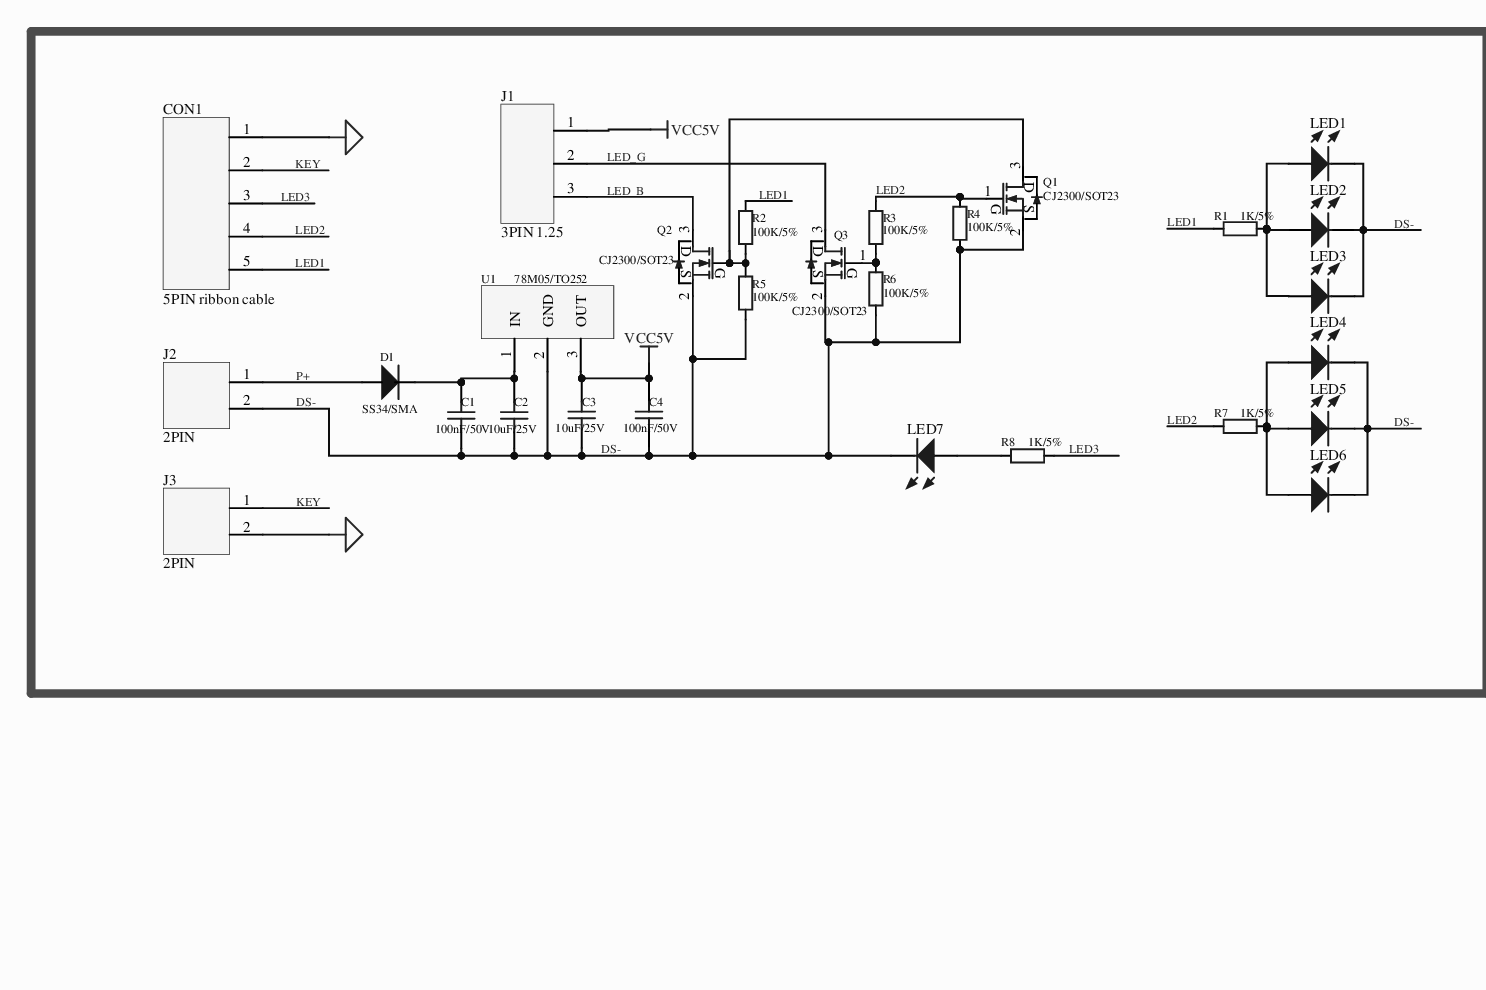
[diagram p0: MISC88840.SchDoc, top left]
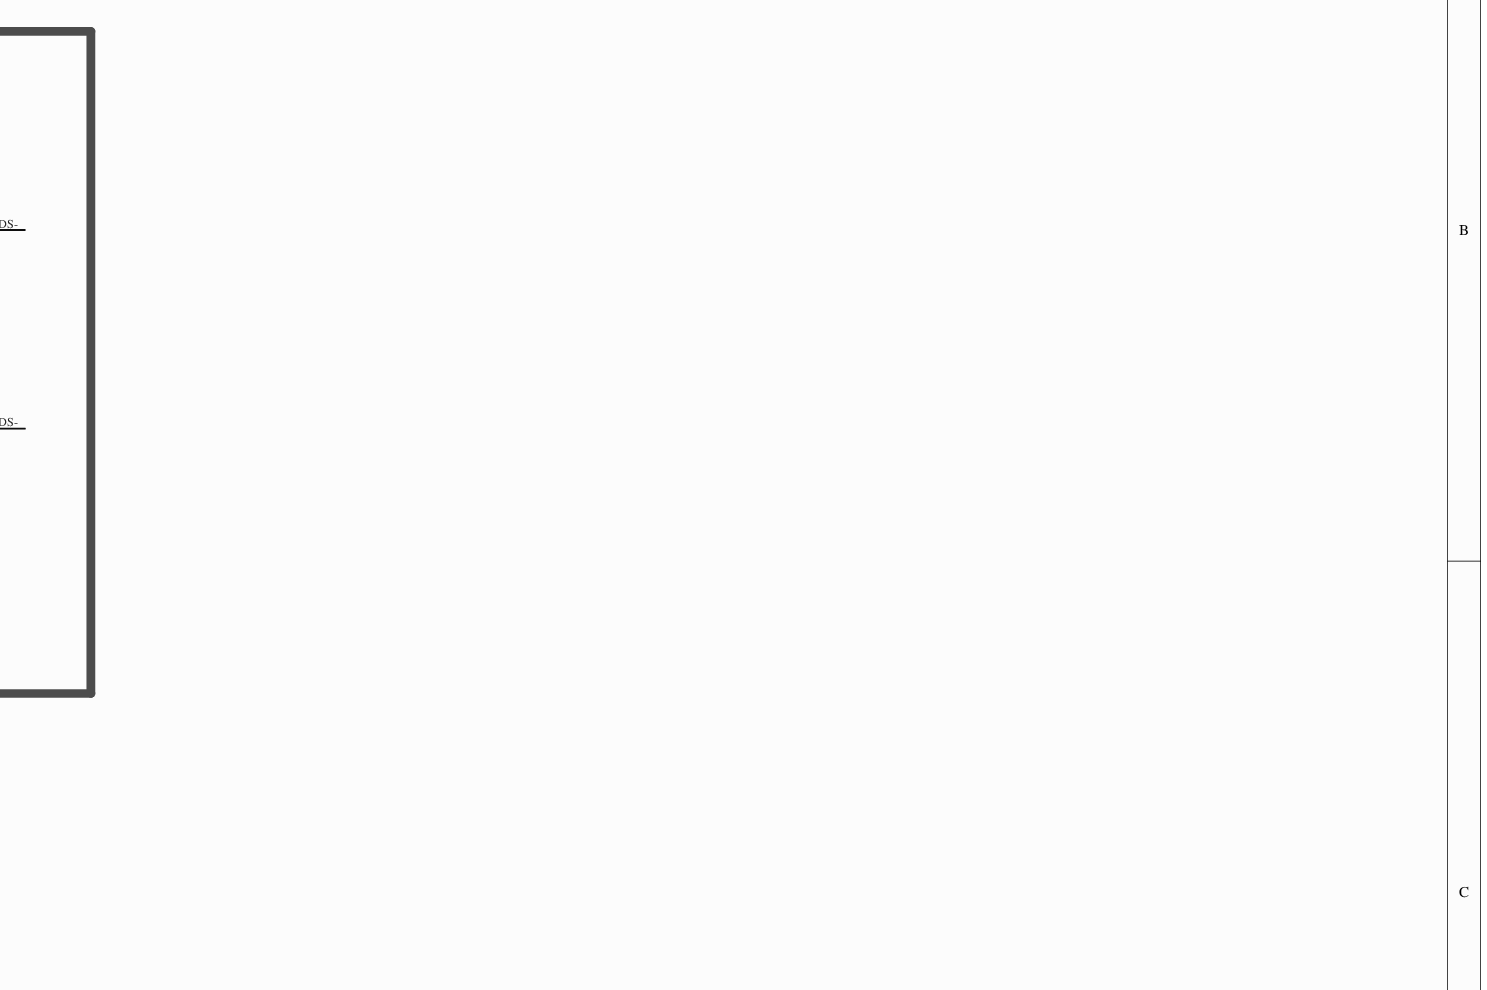
[diagram p1: MISC88840.SchDoc, top right]
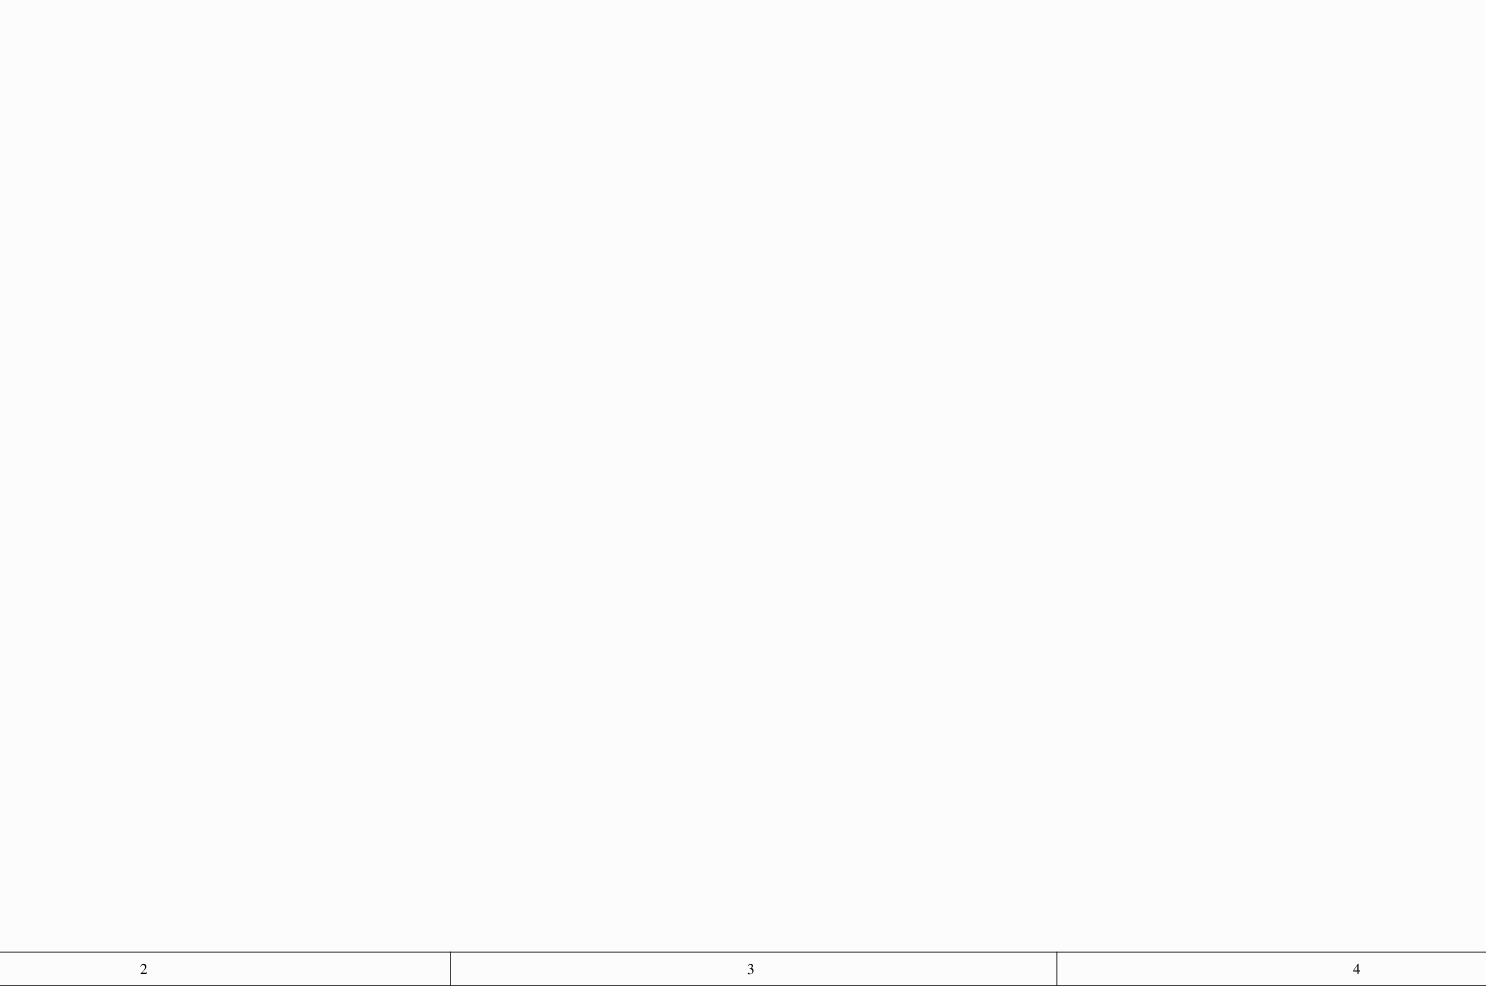
[diagram p2: MISC88840.SchDoc, bottom left]
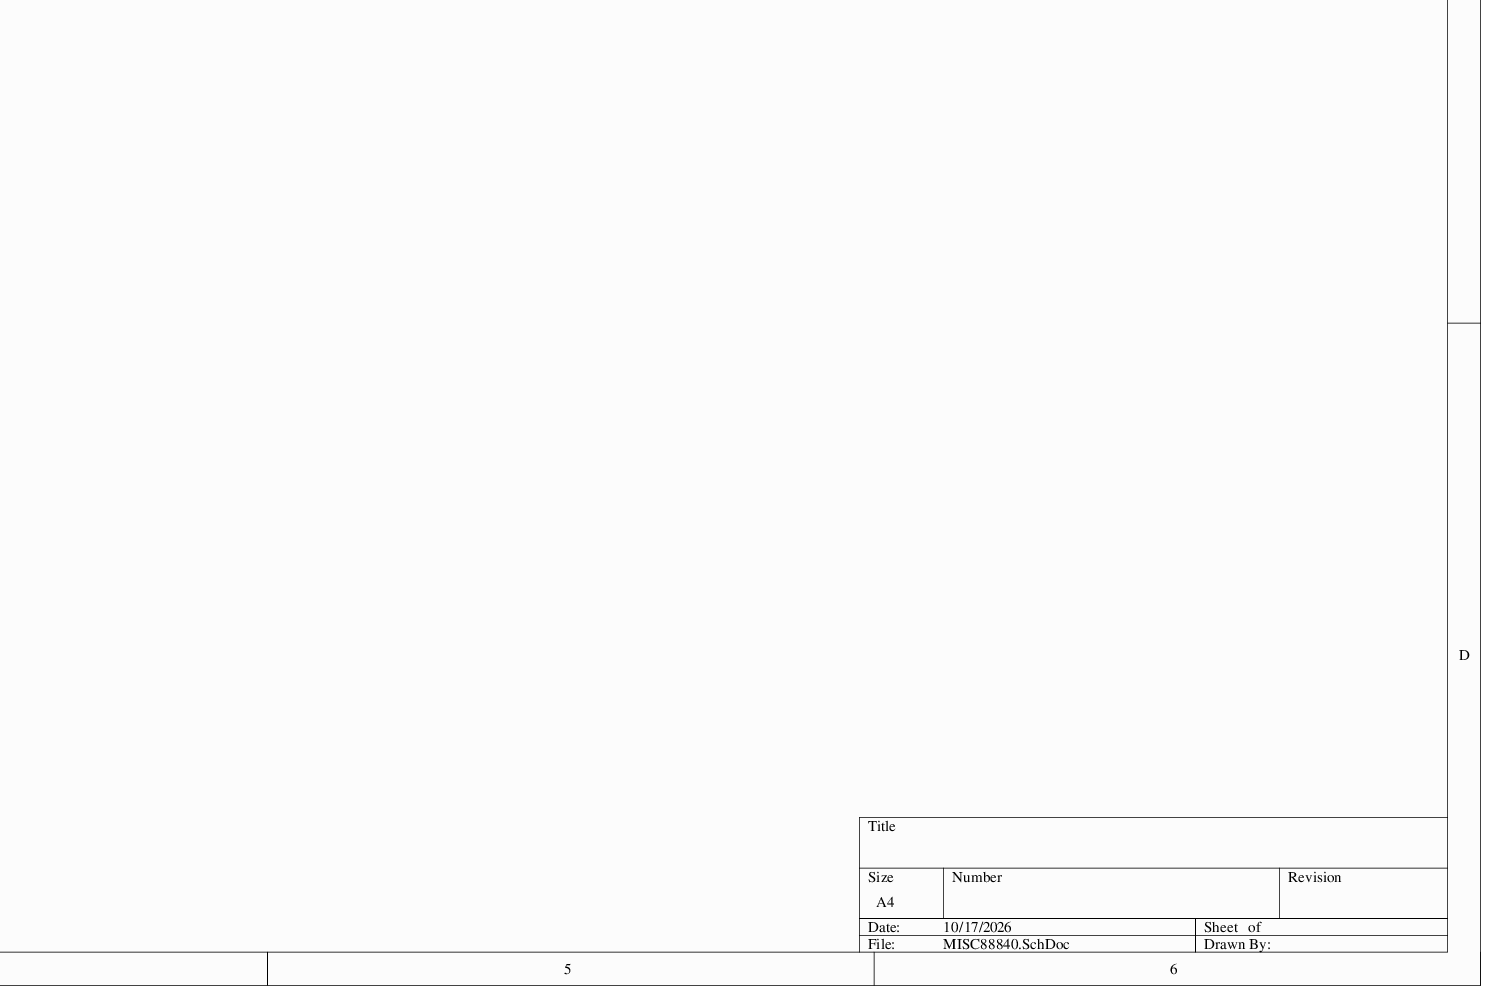
[diagram p3: MISC88840.SchDoc, bottom right]
# Altium project MISC88840.PrjPcb
1 sheet, 28 parts. Net scope: global (net labels, ports and power ports of the same name join across sheets).
Board file: MISC88840.PcbDoc

## Sheet MISC88840.SchDoc
size 549 x 400 mm; SheetNumber: 1; SheetTotal: 1

### Parts
C1  100nF/50V  [C0603A]
C2  10uF/25V  [C0805A]
C3  10uF/25V  [C0805A]
C4  100nF/50V  [C0603A]
CON1  5PIN ribbon cable  [GH1.25-5PIN立贴带扣耐温260℃]
D1  SS34/SMA  [SOD323]
J1  3PIN 1.25  [GH1.25-3PIN立贴带扣耐温260℃]
J2  2PIN  [HY2.0WT-2A/P 立贴带扣耐温260℃]
J3  2PIN  [GH1.25-2PIN立贴带扣耐温260℃]
LED1  (no value)  [LED0603A]
LED2  (no value)  [LED0603A]
LED3  (no value)  [LED0603A]
LED4  (no value)  [LED0603A]
LED5  (no value)  [LED0603A]
LED6  (no value)  [LED0603A]
LED7  (no value)  [LED0603A]
Q1  CJ2300/SOT23  [SOT-23-3 MOS]
Q2  CJ2300/SOT23  [SOT-23-3 MOS]
Q3  CJ2300/SOT23  [SOT-23-3 MOS]
R1  1K/5%  [R0603A]
R2  100K/5%  [R0603A]
R3  100K/5%  [R0603A]
R4  100K/5%  [R0603A]
R5  100K/5%  [R0603A]
R6  100K/5%  [R0603A]
R7  1K/5%  [R0603A]
R8  1K/5%  [R0603A]
U1  78M05/TO252  [TO-252-A]

### Nets
B-: CON1.1 J3.2
VCC5V: C3.2 C4.2 J1.1 U1.3(OUT)
DS-: C1.1 C2.1 C3.1 C4.1 J2.2 LED1.2 LED2.2 LED3.2 LED4.2 LED5.2 LED6.2 LED7.2 Q1.2(S) Q2.2(S) Q3.2(S) R4.2 R5.1 R6.1 U1.2(GND)
KEY: CON1.2 J3.1
LED1: CON1.5 R1.1 R2.1
LED2: CON1.4 Q1.1(G) R3.1 R4.1 R7.1
LED3: CON1.3 R8.2
LED_B: J1.3 Q2.3(D)
LED_G: J1.2 Q3.3(D)
P+: D1.1 J2.1
NetC1_2: C1.2 C2.2 D1.2 U1.1(IN)
NetLED1_1: LED1.1 LED2.1 LED3.1 R1.2
NetLED4_1: LED4.1 LED5.1 LED6.1 R7.2
NetLED7_1: LED7.1 R8.1
NetQ1_3: Q1.3(D) Q2.1(G) R2.2 R5.2
NetQ3_1: Q3.1(G) R3.2 R6.2

### Library data of the parts
C1 C4 = C0603: SMD capacitor
C2 C3 = C0805: SMD capacitor
CON1 = 5PIN: 10PIN dual row
D1 = T4: Fast recovery diode; 物料名称: 4148; 封装: SOD323
J1 = 3PIN: DC socket 3PIN, 2.0 pitch; 封装: 90° right angle, 2.0 pitch; 物料名称: DC socket 3PIN
J2 J3 = 2PIN: DC socket right angle 90°, 2.0 pitch; 物料名称: DC socket 2PIN; 封装: 2.0 pitch 90° right angle
LED1-LED7 = LED 白发蓝: SMD LED; 规格: 0603-diffused-ice blue
Q1-Q3 = MOS-N: Single N-channel MOSFET
R1-R8 = Res0603: SMD resistor; 规格: 0603
U1 = HT7533_SO89: SMD LDO